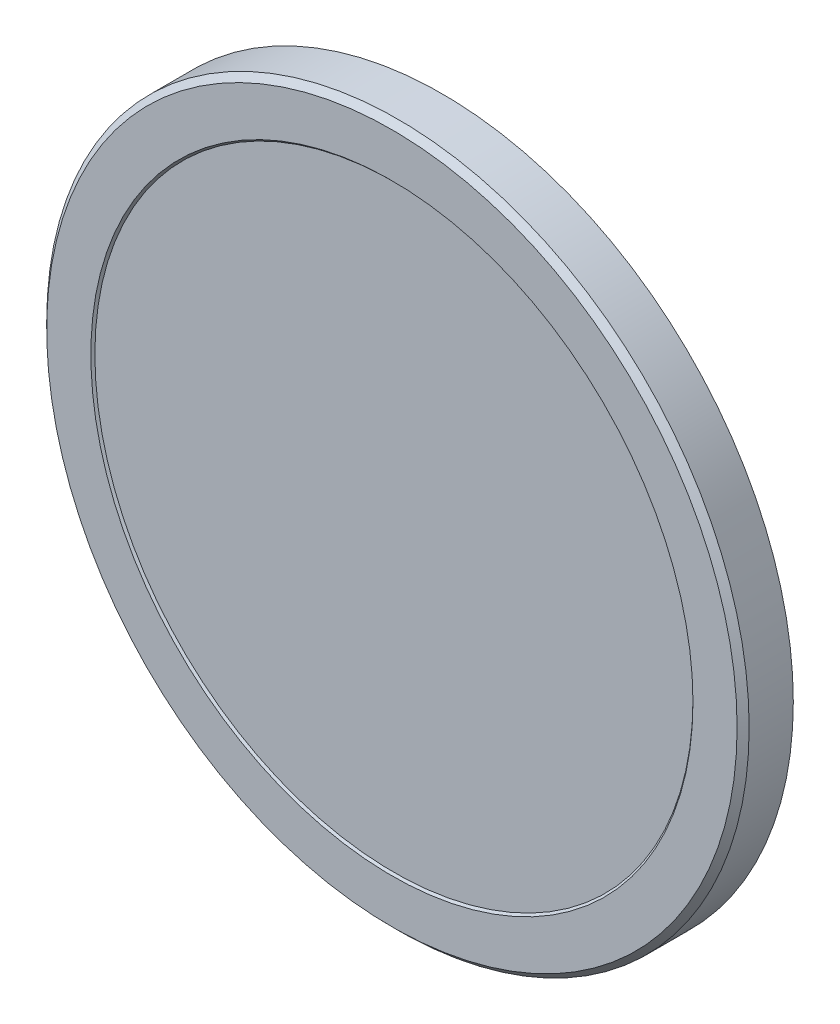
SolidWorks part; units mm, degrees
ref_plane "Front Plane" through (0, 0, 0) normal (0, 0, 1) x (1, 0, 0)
ref_plane "Top Plane" through (0, 0, 0) normal (0, 1, 0) x (1, 0, 0)
ref_plane "Right Plane" through (0, 0, 0) normal (1, 0, 0) x (0, 0, -1)
sketch "Sketch1" plane through (0, 0, 0) normal (0, 0, 1) x (1, 0, 0)
  circle A0 centre (0, 0) radius 34
  dimension "D1" = 68
extrude "Boss-Extrude1" add sketch "Sketch1" along normal blind 50
sketch "Sketch2" plane through (0, 0, 50) normal (0, 0, 1) x (1, 0, 0)
  circle A0 centre (0, 0) radius 175
  dimension "D1" = 350
extrude "Boss-Extrude2" add sketch "Sketch2" against normal blind 25
sketch "Sketch3" plane through (0, 0, 50) normal (0, 0, 1) x (1, 0, 0)
  circle A0 centre (0, 0) radius 150
  dimension "D1" = 300
extrude "Cut-Extrude1" cut sketch "Sketch3" against normal blind 1 draft 45
fillet "Fillet1" radius 0.5 1 edges at (34, 0, 25)
chamfer "Chamfer1" distance 3 angle 45 1 edges at (175, 0, 50)
